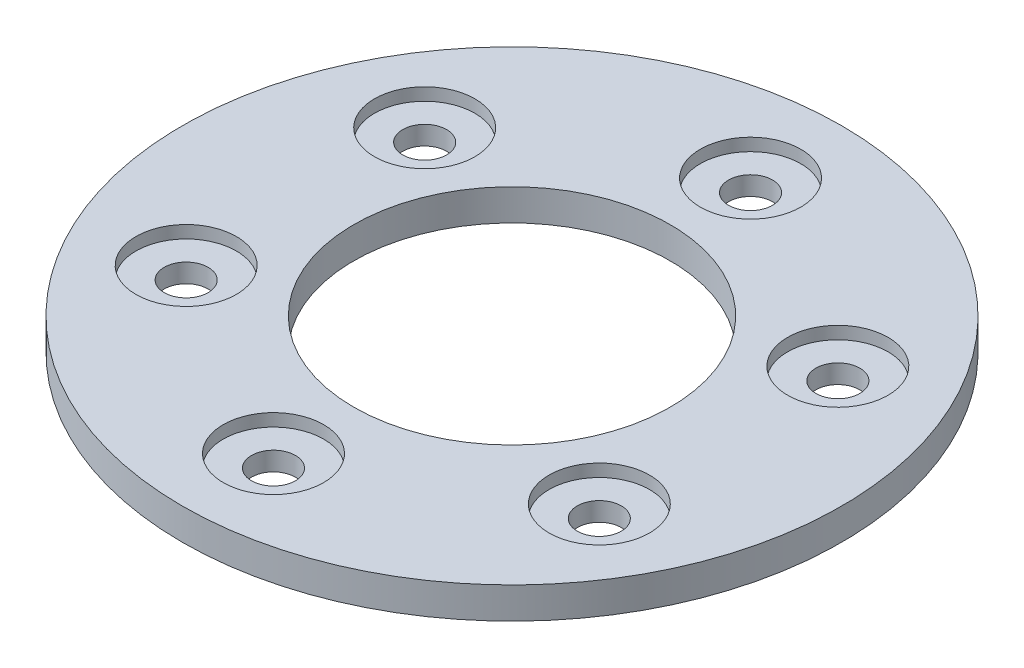
from build123d import *

# Parameters (mm, degrees)
SKETCH1_R           = 26.25
SKETCH1_R_2         = 12.6
BOSS_EXTRUDE1_DEPTH = 4
SKETCH2_R           = 35
SKETCH2_R_2         = 14.25
CUT_EXTRUDE1_DEPTH  = 1.5
SKETCH4_R           = 1.75
CUT_EXTRUDE2_DEPTH  = 10
CIRPATTERN1_COUNT   = 6
SKETCH5_R           = 4
CUT_EXTRUDE3_DEPTH  = 1
CIRPATTERN2_COUNT   = 6
CHAMFER1_SIZE       = 0.5
SKETCH6_R           = 14.25
CUT_EXTRUDE4_DEPTH  = 1.5


with BuildPart() as part:
    # Sketch1 → Boss-Extrude1 (new body)
    with BuildSketch(Plane(origin=(0, 0, 0), x_dir=(1, 0, 0), z_dir=(0, 1, 0))):
        with Locations(Location((0, 0, 0), (0, 0, 270))):
            Circle(SKETCH1_R)
        with Locations(Location((0, 0, 0), (0, 0, 270))):
            Circle(SKETCH1_R_2, mode=Mode.SUBTRACT)
    extrude(amount=BOSS_EXTRUDE1_DEPTH)

    # Sketch2 → Cut-Extrude1 (cut)
    with BuildSketch(Plane(origin=(0, 4, 0), x_dir=(1, 0, 0), z_dir=(0, 1, 0))):
        Circle(SKETCH2_R)
        with Locations(Location((0, 0, 0), (0, 0, 270))):
            Circle(SKETCH2_R_2, mode=Mode.SUBTRACT)
    extrude(amount=-CUT_EXTRUDE1_DEPTH, mode=Mode.SUBTRACT)

    # Sketch4 → Cut-Extrude2 (cut)
    with BuildSketch(Plane(origin=(0, 2.5, 0), x_dir=(1, 0, 0), z_dir=(0, 1, 0))):
        with Locations(Location((0, 19, 0), (0, 0, 270))):
            Circle(SKETCH4_R)
    cut_extrude2 = extrude(amount=-CUT_EXTRUDE2_DEPTH, mode=Mode.SUBTRACT)

    # CirPattern1: Cut-Extrude2 ×6 about axis
    cirpattern1_axis = Axis((0, 0, 0), (0, 1, 0))
    for i in range(1, CIRPATTERN1_COUNT):
        add(cut_extrude2.rotate(cirpattern1_axis, i * 360 / CIRPATTERN1_COUNT), mode=Mode.SUBTRACT)

    # Sketch5 → Cut-Extrude3 (cut)
    with BuildSketch(Plane(origin=(0, 2.5, 0), x_dir=(1, 0, 0), z_dir=(0, 1, 0))):
        with Locations(Location((0, 19, 0), (0, 0, 270))):
            Circle(SKETCH5_R)
    cut_extrude3 = extrude(amount=-CUT_EXTRUDE3_DEPTH, mode=Mode.SUBTRACT)

    # CirPattern2: Cut-Extrude3 ×6 about axis
    cirpattern2_axis = Axis((0, 0, 0), (0, 1, 0))
    for i in range(1, CIRPATTERN2_COUNT):
        add(cut_extrude3.rotate(cirpattern2_axis, i * 360 / CIRPATTERN2_COUNT), mode=Mode.SUBTRACT)

    # Chamfer1
    chamfer1_edges = [part.edges().sort_by_distance(p)[0] for p in [
        (0, 4, -14.25),
    ]]
    chamfer(chamfer1_edges, length=CHAMFER1_SIZE)

    # Sketch6 → Cut-Extrude4 (cut)
    with BuildSketch(Plane(origin=(0, 4, 0), x_dir=(1, 0, 0), z_dir=(0, 1, 0))):
        Circle(SKETCH6_R)
    extrude(amount=-CUT_EXTRUDE4_DEPTH, mode=Mode.SUBTRACT)


solid = part.part
